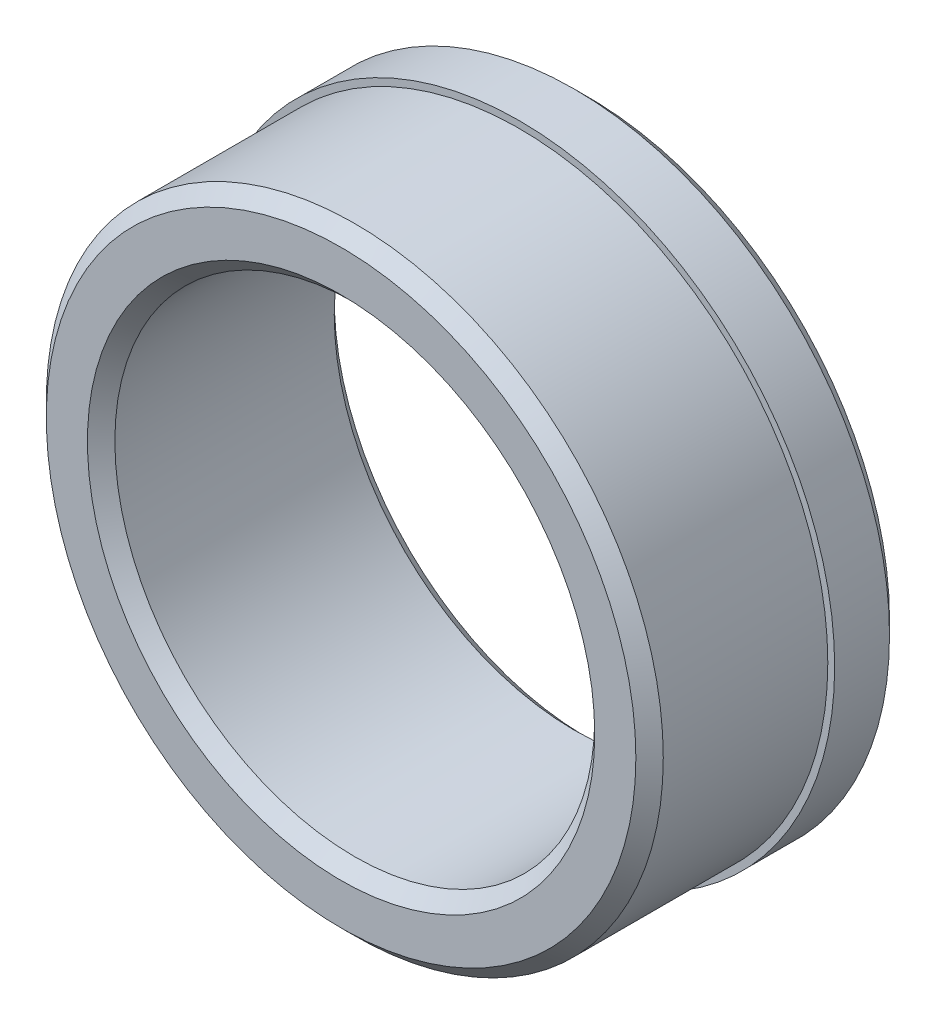
from build123d import *

# Parameters (mm, degrees)
SKETCH1_W     = 26
SKETCH1_H     = 10
CHAMFER1_SIZE = 2


with BuildPart() as part:
    # Sketch1 → Revolve1 (revolve)
    with BuildSketch(Plane(origin=(0, 0, 0), x_dir=(0, 0, -1), z_dir=(1, 0, 0)), mode=Mode.PRIVATE) as revolve1_sk:
        with Locations((13, 40)):
            Rectangle(SKETCH1_W, SKETCH1_H)
        Polygon((26, 45), (26, 35), (36, 35), (36, 46), (26, 46), align=None)
    revolve(revolve1_sk.sketch.rotate(Axis((0, 0, 0), (0, 0, -1)), 90), axis=Axis((0, 0, 0), (0, 0, -1)))

    # Chamfer1
    chamfer1_edges = [part.edges().sort_by_distance(p)[0] for p in [
        (-45, 0, 0),
        (-46, 0, -36),
        (-35, 0, -36),
        (-35, 0, 0),
    ]]
    chamfer(chamfer1_edges, length=CHAMFER1_SIZE)


solid = part.part
